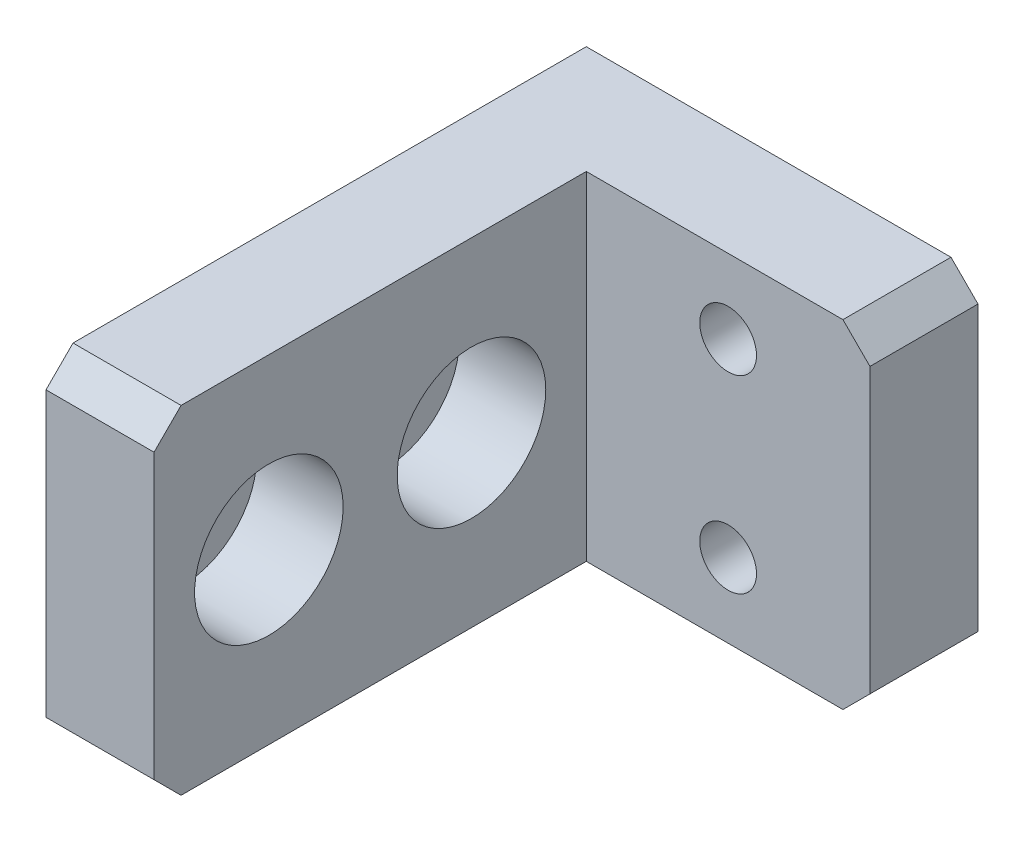
SolidWorks part; units mm, degrees
material "6061Al"
ref_plane "前视基准面" through (0, 0, 0) normal (0, 0, 1) x (1, 0, 0)
ref_plane "上视基准面" through (0, 0, 0) normal (0, 1, 0) x (1, 0, 0)
ref_plane "右视基准面" through (0, 0, 0) normal (1, 0, 0) x (0, 0, -1)
sketch "草图1" plane through (0, 0, 0) normal (0, 1, 0) x (1, 0, 0)
  line L0 (0, 0) -> (0, 32)
  line L1 (0, 32) -> (21, 32)
  line L2 (21, 32) -> (21, 40)
  line L3 (21, 40) -> (-8, 40)
  line L4 (-8, 40) -> (-8, 0)
  line L5 (-8, 0) -> (0, 0)
  dimension "D1" = 29
  dimension "D2" = 8
  dimension "D3" = 8
  dimension "D4" = 40
extrude "凸台-拉伸1" add sketch "草图1" along normal mid plane 25
hole_wizard "M5 螺纹孔1" positions "草图2" profile "草图3" tap size "M5" standard "ISO" end condition through all
sketch "草图2" plane through (0, 0, -32) normal (0, 0, 1) x (1, 0, 0)
  line L0 (0, 0) -> (21, 0) construction
  line L1 (0, 12.5) -> (0, -12.5) construction
  line L2 (21, 12.5) -> (21, -12.5) construction
  line L5 (10.5, 0) -> (10.5, 19.9222) construction
  point P0 (10.5, 7)
  point P2 (10.5, -7)
  dimension "D1" = 14
sketch "草图3" plane through (10.5, 7, -32) normal (1, 0, 0) x (0, -1, 0)
  line L0 (0, 0) -> (0, 8)
  line L1 (0, 8) -> (2.1, 8)
  line L2 (2.1, 8) -> (2.1, 0)
  line L5 (2.1, 0) -> (0, 0)
  line L11 (0, -6.35) -> (0, 107.95) construction
  dimension "通孔螺纹孔钻头直径" = 4.2
  dimension "通孔螺纹孔钻头深度" = 8
hole_wizard "M6 六角凹头螺钉的柱形沉头孔1" positions "草图4" profile "草图5" counterbore size "M6" standard "ISO" end condition through all
sketch "草图4" plane through (0, 0, 0) normal (1, 0, 0) x (0, 0, -1)
  line L0 (0, 0) -> (32, 0) construction
  line L1 (32, 12.5) -> (32, -12.5) construction
  line L3 (0, 12.5) -> (0, -12.5) construction
  point P0 (8.5, 0)
  point P2 (23.5, 0)
  dimension "D1" = 8.5
  dimension "D2" = 15
sketch "草图5" plane through (0, 0, -8.5) normal (0, 1, 0) x (0, 0, -1)
  line L0 (0, 0) -> (0, 8)
  line L1 (0, 8) -> (3.3, 8)
  line L3 (3.3, 8) -> (3.3, 6.4)
  line L4 (3.3, 6.4) -> (5.5, 6.4)
  line L5 (5.5, 6.4) -> (5.5, 0)
  line L7 (5.5, 0) -> (0, 0)
  line L11 (0, -6.35) -> (0, 107.95) construction
  dimension "通孔孔直径" = 6.6
  dimension "通孔孔深度" = 8
  dimension "柱形沉头孔直径" = 11
  dimension "柱形沉头孔深度" = 6.4
chamfer "倒角1" distance 2 angle 45 4 edges at (-4, 12.5, 0) (-4, -12.5, 0) (21, -12.5, -36) (21, 12.5, -36)
